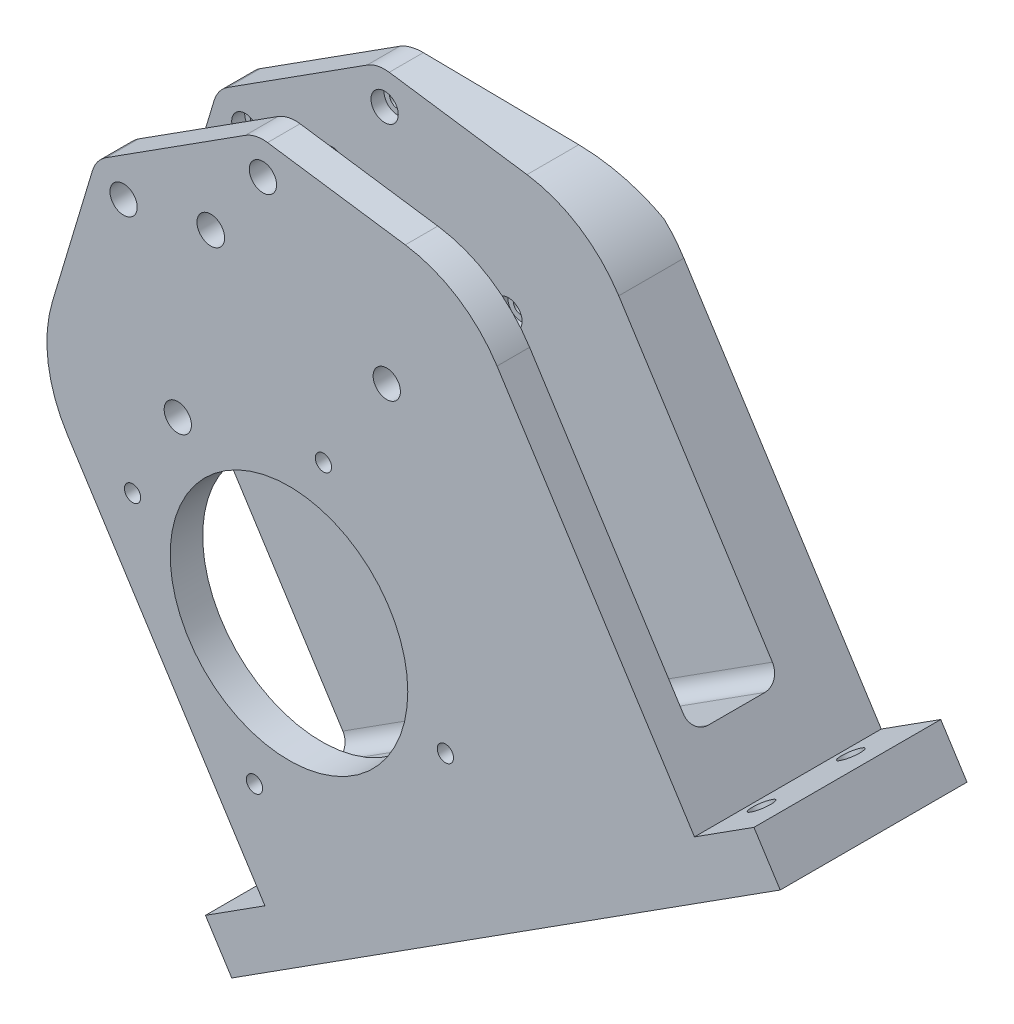
from build123d import *

# Parameters (mm, degrees)
SKETCH_1_R             = 4.191
EXTRUDE_1_DEPTH        = 10
SKETCH_2_R             = 2.5
CUT_EXTRUDE_1_DEPTH    = 10
SKETCH_3_W             = 156.633333356
SKETCH_3_H             = 10
EXTRUDE_2_DEPTH        = 22.68
SKETCH_4_R             = 36.51
CUT_EXTRUDE_2_DEPTH    = 215.91006095
HOLE_WIZARD_M6_1_D     = 5
EXTRUDE_3_DEPTH        = 156.633333356
CUT_EXTRUDE_3_DEPTH    = 238.627708353
CUT_EXTRUDE_START      = -4
SKETCH_10_R            = 4.191
CUT_EXTRUDE_4_DEPTH    = 4
HOLE_WIZARD_M6_2_D     = 5
FILLET_2_R             = 5
EXTRUDE_4_DEPTH        = 57.4
SKETCH_14_R            = 4.25
CUT_EXTRUDE_5_DEPTH    = 274.867467739
HOLE_WIZARD_M8_1_D     = 6.8
HOLE_WIZARD_M8_2_D     = 6.8
HOLE_WIZARD_M8_2_DEPTH = 19.75
HOLE_WIZARD_M8_2_TIP   = 2.042926105
MM_1_D                 = 10
MM_1_DEPTH             = 19.75
MM_1_TIP               = 3.004303095


with BuildPart() as part:
    # 草图1 → 凸台-拉伸1 (new body)
    with BuildSketch(Plane.XY):
        with BuildLine():
            Line((-48.192429183, -18.924316881), (-5.38408585, 8.426839239))
            ThreePointArc((-5.38408585, 8.426839239), (-2.115871946, 9.773591249), (1.416719377, 9.899136639))
            Line((1.416719377, 9.899136639), (43.750815051, 3.840473561))
            ThreePointArc((43.750815051, 3.840473561), (59.829864165, -2.159919824), (71.943180436, -14.317555701))
            Line((71.943180436, -14.317555701), (109.631781388, -73.305430372))
            Line((109.631781388, -73.305430372), (-22.360610574, -157.638161754))
            Line((-22.360610574, -157.638161754), (-60.049211526, -98.650287083))
            ThreePointArc((-60.049211526, -98.650287083), (-65.990843282, -82.549431417), (-64.6787621, -65.437476996))
            Line((-64.6787621, -65.437476996), (-52.386334807, -24.476772825))
            ThreePointArc((-52.386334807, -24.476772825), (-50.787903547, -21.323999346), (-48.192429183, -18.924316881))
        make_face()
        with Locations((-26.159273046, -76.997288483)):
            Circle(SKETCH_1_R, mode=Mode.SUBTRACT)
        with Locations((38.053241953, -35.970554303)):
            Circle(SKETCH_1_R, mode=Mode.SUBTRACT)
        Circle(SKETCH_1_R, mode=Mode.SUBTRACT)
        with Locations((-42.808343333, -27.35115612)):
            Circle(SKETCH_1_R, mode=Mode.SUBTRACT)
    extrude(amount=EXTRUDE_1_DEPTH)

    # 草图2 → 切除-拉伸1 (cut)
    with BuildSketch(Plane(origin=(0, 0, 0), x_dir=(-1, 0, 0), z_dir=(0, 0, -1))):
        with Locations((-8.003999953, -114.717481812)):
            Circle(SKETCH_2_R)
    extrude(amount=-CUT_EXTRUDE_1_DEPTH, mode=Mode.SUBTRACT)

    # 草图3 → 凸台-拉伸2 (add)
    with BuildSketch(Plane(origin=(65.039757073, -101.796218004, 0), x_dir=(0.8426839238753957, 0.538408585037392, 0), z_dir=(0.538408585037392, -0.8426839238753957, 0))):
        with Locations((-25.399999999, 5)):
            Rectangle(SKETCH_3_W, SKETCH_3_H)
    extrude(amount=EXTRUDE_2_DEPTH)

    # 草图4 → 切除-拉伸2 (cut, through all)
    with BuildSketch(Plane.XY.offset(10)):
        with Locations((8.003999953, -114.717481812)):
            Circle(SKETCH_4_R)
    extrude(amount=-CUT_EXTRUDE_2_DEPTH, mode=Mode.SUBTRACT)

    # M6 螺纹孔1 (through all)
    with Locations(Plane.XY.offset(10)):
        with Locations((-2.584781838, -162.779501122), (-40.058019357, -104.128700021), (56.066019263, -125.306263604), (18.592781745, -66.655462502)):
            Hole(HOLE_WIZARD_M6_1_D / 2)

    # 草图7 → 凸台-拉伸3 (add)
    with BuildSketch(Plane(origin=(-87.400367646, -55.84194375, 0), x_dir=(0, 0, 1), z_dir=(-0.8426839238753956, -0.5384085850373922, 0))):
        Polygon((-27.4, -143.48), (10, -143.48), (10, -163.48), (-47.4, -163.48), (-47.4, -41.275), (-37.4, 10), (-27.4, 10), align=None)
    extrude(amount=-EXTRUDE_3_DEPTH)

    # 草图8 → 切除-拉伸3 (cut, through all)
    with BuildSketch(Plane.XY.offset(-27.4)):
        with BuildLine():
            Line((71.943180436, -14.317555701), (39.207938465, 36.91762687))
            Line((39.207938465, 36.91762687), (-7.989717867, 44.981113167))
            Line((-7.989717867, 44.981113167), (-89.961386524, -17.397404979))
            Line((-89.961386524, -17.397404979), (-92.784453497, -47.415104511))
            Line((-92.784453497, -47.415104511), (-60.049211526, -98.650287083))
            ThreePointArc((-60.049211526, -98.650287083), (-65.990843282, -82.549431417), (-64.6787621, -65.437476996))
            Line((-64.6787621, -65.437476996), (-52.386334807, -24.476772825))
            ThreePointArc((-52.386334807, -24.476772825), (-50.787903547, -21.323999346), (-48.192429183, -18.924316881))
            Line((-48.192429183, -18.924316881), (-5.38408585, 8.426839239))
            ThreePointArc((-5.38408585, 8.426839239), (-2.115871946, 9.773591249), (1.416719377, 9.899136639))
            Line((1.416719377, 9.899136639), (43.750815051, 3.840473561))
            ThreePointArc((43.750815051, 3.840473561), (59.829864165, -2.159919824), (71.943180436, -14.317555701))
        make_face()
    extrude(amount=-CUT_EXTRUDE_3_DEPTH, mode=Mode.SUBTRACT)

    # 草图10 → 切除-拉伸4 (cut)
    with BuildSketch(Plane.XY.offset(-27.4).offset(CUT_EXTRUDE_START)):
        with Locations((38.053241953, -35.970554303)):
            Circle(SKETCH_10_R)
        with Locations((-26.159273046, -76.997288483)):
            Circle(SKETCH_10_R)
        with Locations((-42.808343333, -27.35115612)):
            Circle(SKETCH_10_R)
        Circle(SKETCH_10_R)
    extrude(amount=CUT_EXTRUDE_4_DEPTH, mode=Mode.SUBTRACT)

    # M6 螺纹孔2 (through all)
    with Locations(Plane.XY.offset(-31.4)):
        with Locations((0, 0), (38.053241953, -35.970554303), (-26.159273046, -76.997288483), (-42.808343333, -27.35115612)):
            Hole(HOLE_WIZARD_M6_2_D / 2)

    # 圆角2
    fillet_2_edges = [part.edges().sort_by_distance(p)[0] for p in [
        (55.846692116, -134.583867457, 0),
        (55.846692116, -134.583867457, -27.4),
    ]]
    fillet(fillet_2_edges, radius=FILLET_2_R)

    # 草图13 → 凸台-拉伸4 (add)
    with BuildSketch(Plane.XY.offset(10)):
        Polygon((150.883256204, -97.596687431), (-17.653528571, -205.278404438), (-9.577399795, -217.918663296), (158.95938498, -110.236946289), align=None)
    extrude(amount=-EXTRUDE_4_DEPTH)

    # 草图14 → 切除-拉伸5 (cut, through all)
    with BuildSketch(Plane(origin=(0, 0, 0), x_dir=(-1, 0, 0), z_dir=(0, 0, -1))):
        with Locations((16.020085816, -22.102417299)):
            Circle(SKETCH_14_R)
    extrude(amount=-CUT_EXTRUDE_5_DEPTH, mode=Mode.SUBTRACT)

    # M8 螺纹孔1 (through all)
    with Locations(Plane.XY.offset(-27.4)):
        with Locations((-16.020085816, -22.102417299)):
            Hole(HOLE_WIZARD_M8_1_D / 2)

    # M8 螺纹孔2
    with Locations(Plane(origin=(96.095164257, -150.402226733, 0), x_dir=(-0.8426839238753955, -0.538408585037392, 0), z_dir=(0.5384085850373921, -0.8426839238753956, 0))):
        with Locations((110.399999999, 5), (110.399999999, 32.4), (-59.600000001, 32.4), (-59.600000001, 5)):
            Hole(HOLE_WIZARD_M8_2_D / 2, depth=HOLE_WIZARD_M8_2_DEPTH)
            with Locations((0, 0, -(HOLE_WIZARD_M8_2_DEPTH + HOLE_WIZARD_M8_2_TIP / 2))):  # 118° drill point
                Cone(0, HOLE_WIZARD_M8_2_D / 2, HOLE_WIZARD_M8_2_TIP, mode=Mode.SUBTRACT)

    # 大小mm 暗销孔1
    with Locations(Plane(origin=(96.095164257, -150.402226733, 0), x_dir=(-0.8426839238753955, -0.538408585037392, 0), z_dir=(0.5384085850373921, -0.8426839238753956, 0))):
        with Locations((65.399999999, 18.7), (-14.600000001, 18.7)):
            Hole(MM_1_D / 2, depth=MM_1_DEPTH)
            with Locations((0, 0, -(MM_1_DEPTH + MM_1_TIP / 2))):  # 118° drill point
                Cone(0, MM_1_D / 2, MM_1_TIP, mode=Mode.SUBTRACT)


solid = part.part
